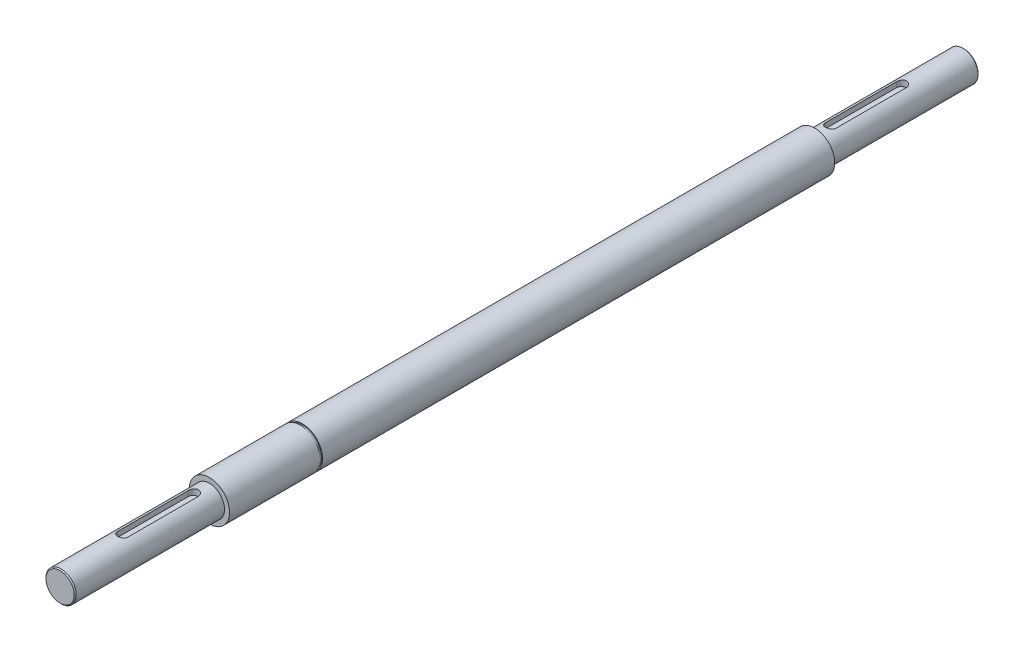
SolidWorks part; units mm, degrees
material "普通碳钢"
ref_plane "前视基准面" through (0, 0, 0) normal (0, 0, 1) x (1, 0, 0)
ref_plane "上视基准面" through (0, 0, 0) normal (0, 1, 0) x (1, 0, 0)
ref_plane "右视基准面" through (0, 0, 0) normal (1, 0, 0) x (0, 0, -1)
sketch "草图1" plane through (0, 0, 0) normal (0, 0, 1) x (1, 0, 0)
  circle A1 centre (0, 0) radius 10
  dimension "D2" = 20
extrude "凸台-拉伸1" add sketch "草图1" along normal blind 300
sketch "草图2" plane through (0, 0, 0) normal (0, 0, -1) x (-1, 0, 0)
  circle A0 centre (0, 0) radius 6
  dimension "D1" = 12
extrude "凸台-拉伸2" add sketch "草图2" along normal blind 74
sketch "草图3" plane through (0, 0, 300) normal (0, 0, 1) x (1, 0, 0)
  circle A0 centre (0, 0) radius 6
  dimension "D1" = 12
extrude "凸台-拉伸3" add sketch "草图3" along normal blind 74
ref_plane "基准面1" through (0, 7.5, 0) normal (0, 1, 0) x (1, 0, 0)
sketch "草图4" plane through (0, 0, 300) normal (0, 0, 1) x (1, 0, 0)
  circle A0 centre (0, 0) radius 7.5
  dimension "D1" = 15
extrude "凸台-拉伸4" add sketch "草图4" along normal blind 74
sketch "草图5" plane through (0, 0, 0) normal (0, 0, -1) x (-1, 0, 0)
  circle A0 centre (0, 0) radius 7.5
  dimension "D1" = 15
extrude "凸台-拉伸5" add sketch "草图5" along normal blind 74
sketch "草图7" plane through (0, 7.5, 0) normal (0, 1, 0) x (1, 0, 0)
  line L0 (0, 0) -> (0, 116.1752) construction
  line L1 (0, 8) -> (0, 43) construction
  line L2 (-2.5, 8) -> (-2.5, 43)
  line L3 (2.5, 8) -> (2.5, 43)
  line L4 (10, 0) -> (-10, 0) construction
  line L5 (0, -300) -> (0, -349.1508) construction
  line L6 (-7.5, -300) -> (7.5, -300) construction
  line L7 (0, -308) -> (0, -343) construction
  line L8 (2.5, -308) -> (2.5, -343)
  line L9 (-2.5, -308) -> (-2.5, -343)
  arc A0 (-2.5, 8) -> (2.5, 8) centre (0, 8) ccw
  arc A1 (2.5, 43) -> (-2.5, 43) centre (0, 43) ccw
  arc A2 (2.5, -308) -> (-2.5, -308) centre (0, -308) ccw
  arc A3 (-2.5, -343) -> (2.5, -343) centre (0, -343) ccw
  point P5 (0, 25.5)
  point P18 (0, -325.5)
  dimension "D2" = 2.5
  dimension "D6" = 2.5
  dimension "D1" = 8
  dimension "D3" = 35
  dimension "D4" = 8
  dimension "D5" = 35
extrude "切除-拉伸1" cut sketch "草图7" against normal blind 3
chamfer "倒角1" distance 0.5 angle 45
sketch "草图8" plane through (0, 0, 255) normal (0, 0, -1) x (-1, 0, 0)
  circle A0 centre (0, 0) radius 9.5
  circle A1 centre (0, 0) radius 12.5
  dimension "D1" = 19
  dimension "D2" = 25
extrude "切除-拉伸2" cut sketch "草图8" along normal blind 1.1
